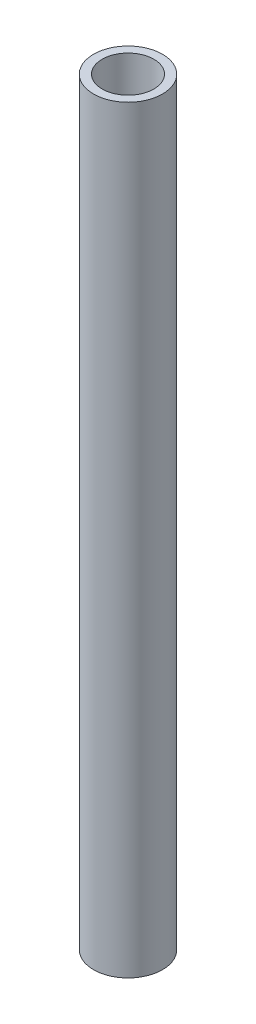
from build123d import *

# Parameters (mm, degrees)
SKETCH1_W = 0.25
SKETCH1_H = 22


with BuildPart() as part:
    # Sketch1 → Revolve1 (revolve)
    with BuildSketch(Plane.XY, mode=Mode.PRIVATE) as revolve1_sk:
        with Locations((-0.875, -0.8)):
            Rectangle(SKETCH1_W, SKETCH1_H)
    revolve(revolve1_sk.sketch.rotate(Axis((0, -14.433529877, 0), (0, 1, 0)), 270), axis=Axis((0, -14.433529877, 0), (0, 1, 0)))


solid = part.part
